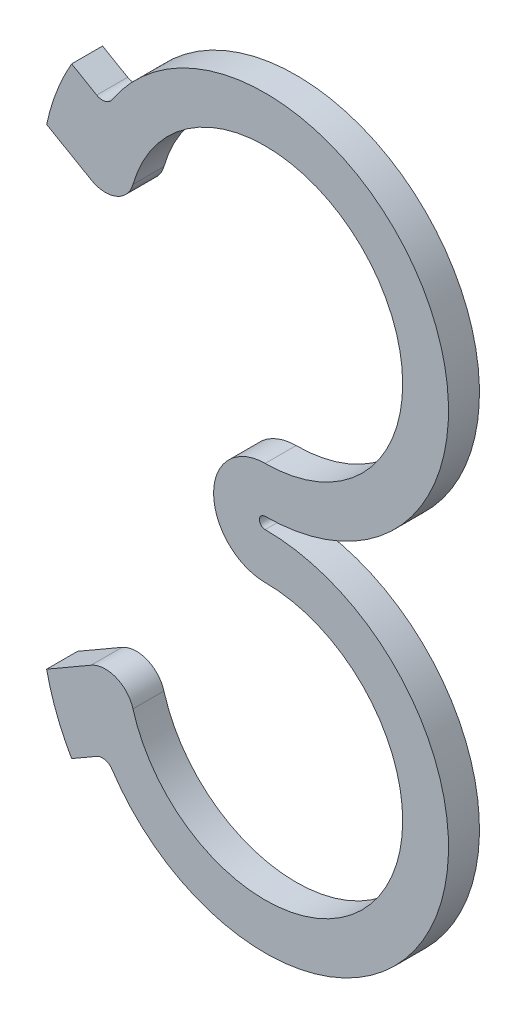
SolidWorks part; units mm, degrees
ref_plane "Front Plane" through (0, 0, 0) normal (0, 0, 1) x (1, 0, 0)
ref_plane "Top Plane" through (0, 0, 0) normal (0, 1, 0) x (1, 0, 0)
ref_plane "Right Plane" through (0, 0, 0) normal (1, 0, 0) x (0, 0, -1)
sketch "Sketch1" plane through (0, 0, 0) normal (0, 0, 1) x (1, 0, 0)
  line L0 (-14.6969, 24.9853) -> (-16.8875, 26.25)
  line L1 (0, 0) -> (76.8643, 0) construction
  line L2 (0, -16.5) -> (0, 16.5) construction
  line L3 (-15.1861, 18.3395) -> (-19.0682, 20.5808)
  line L4 (-3, 11.3038) -> (-16.8564, 19.3038) construction
  line L5 (0, 16.5) -> (-13.8564, 24.5) construction
  line L6 (0, 16.5) -> (-10.3923, 22.5) construction
  line L7 (-10.3923, 22.5) -> (-13.8564, 24.5) construction
  line L8 (-10.3923, -22.5) -> (-13.8564, -24.5) construction
  line L9 (0, -16.5) -> (-10.3923, -22.5) construction
  line L10 (-15.1861, -18.3395) -> (-19.0682, -20.5808)
  line L11 (-14.6969, -24.9853) -> (-16.8875, -26.25)
  arc A0 (0, 4.5) -> (-11.5333, 19.8141) centre (0, 16.5) ccw
  arc A1 (0, 0.5) -> (0, -0.5) centre (0, 0) ccw
  arc A2 (0, 4.5) -> (0, -4.5) centre (0, 0) ccw
  arc A3 (0, 0.5) -> (-13.3618, 25.3012) centre (0, 16.5) ccw
  arc A6 (-11.5333, 19.8141) -> (-15.1861, 18.3395) centre (-13.9361, 20.5045) cw
  arc A8 (-16.8875, 26.25) -> (-19.0682, 20.5808) centre (0, 16.5) ccw
  arc A9 (-13.3618, 25.3012) -> (-14.6969, 24.9853) centre (-14.1969, 25.8513) cw
  arc A10 (-13.3618, -25.3012) -> (-14.6969, -24.9853) centre (-14.1969, -25.8513) ccw
  arc A11 (-16.8875, -26.25) -> (-19.0682, -20.5808) centre (0, -16.5) cw
  arc A12 (-11.5333, -19.8141) -> (-15.1861, -18.3395) centre (-13.9361, -20.5045) ccw
  arc A13 (0, -0.5) -> (-13.3618, -25.3012) centre (0, -16.5) cw
  arc A14 (0, -4.5) -> (-11.5333, -19.8141) centre (0, -16.5) cw
  dimension "D1" = 24
  dimension "D2" = 1
  dimension "D3" = 9
  dimension "D7" = 2.5
  dimension "D8" = 19.5
  dimension "D9" = 1
  dimension "D6" = 60
  dimension "D5" = 6
extrude "Boss-Extrude1" add sketch "Sketch1" along normal blind 2.7
sketch "Sketch2" plane through (0, 0, 2.7) normal (0, 0, 1) x (1, 0, 0)
  line L4 (-19.0682, 20.5808) -> (-15.1861, 18.3395)
  line L5 (-15.1861, -18.3395) -> (-19.0682, -20.5808)
  line L6 (-16.8875, -26.25) -> (-14.6969, -24.9853)
  line L7 (-14.6969, 24.9853) -> (-16.8875, 26.25)
  line L8 (-19.0682, 20.5808) -> (-15.1861, 18.3395)
  line L9 (-15.1861, -18.3395) -> (-19.0682, -20.5808)
  line L10 (-16.8875, -26.25) -> (-14.6969, -24.9853)
  line L11 (-14.6969, 24.9853) -> (-16.8875, 26.25)
  arc A12 (-16.8875, 26.25) -> (-19.0682, 20.5808) centre (0, 16.5) ccw
  arc A13 (-15.1861, 18.3395) -> (-11.5333, 19.8141) centre (-13.9361, 20.5045) ccw
  arc A14 (0, 4.5) -> (-11.5333, 19.8141) centre (0, 16.5) ccw
  arc A15 (0, 4.5) -> (0, -4.5) centre (0, 0) ccw
  arc A16 (-11.5333, -19.8141) -> (0, -4.5) centre (0, -16.5) ccw
  arc A17 (-11.5333, -19.8141) -> (-15.1861, -18.3395) centre (-13.9361, -20.5045) ccw
  arc A18 (-19.0682, -20.5808) -> (-16.8875, -26.25) centre (0, -16.5) ccw
  arc A19 (-13.3618, -25.3012) -> (-14.6969, -24.9853) centre (-14.1969, -25.8513) ccw
  arc A20 (-13.3618, -25.3012) -> (0, -0.5) centre (0, -16.5) ccw
  arc A21 (0, 0.5) -> (0, -0.5) centre (0, 0) ccw
  arc A22 (0, 0.5) -> (-13.3618, 25.3012) centre (0, 16.5) ccw
  arc A23 (-14.6969, 24.9853) -> (-13.3618, 25.3012) centre (-14.1969, 25.8513) ccw
  arc A24 (-16.8875, 26.25) -> (-19.0682, 20.5808) centre (0, 16.5) ccw
  arc A25 (-15.1861, 18.3395) -> (-11.5333, 19.8141) centre (-13.9361, 20.5045) ccw
  arc A26 (0, 4.5) -> (-11.5333, 19.8141) centre (0, 16.5) ccw
  arc A27 (0, 4.5) -> (0, -4.5) centre (0, 0) ccw
  arc A28 (-11.5333, -19.8141) -> (0, -4.5) centre (0, -16.5) ccw
  arc A29 (-11.5333, -19.8141) -> (-15.1861, -18.3395) centre (-13.9361, -20.5045) ccw
  arc A30 (-19.0682, -20.5808) -> (-16.8875, -26.25) centre (0, -16.5) ccw
  arc A31 (-13.3618, -25.3012) -> (-14.6969, -24.9853) centre (-14.1969, -25.8513) ccw
  arc A32 (-13.3618, -25.3012) -> (0, -0.5) centre (0, -16.5) ccw
  arc A33 (0, 0.5) -> (0, -0.5) centre (0, 0) ccw
  arc A34 (0, 0.5) -> (-13.3618, 25.3012) centre (0, 16.5) ccw
  arc A35 (-14.6969, 24.9853) -> (-13.3618, 25.3012) centre (-14.1969, 25.8513) ccw
  dimension "D1" = 0
